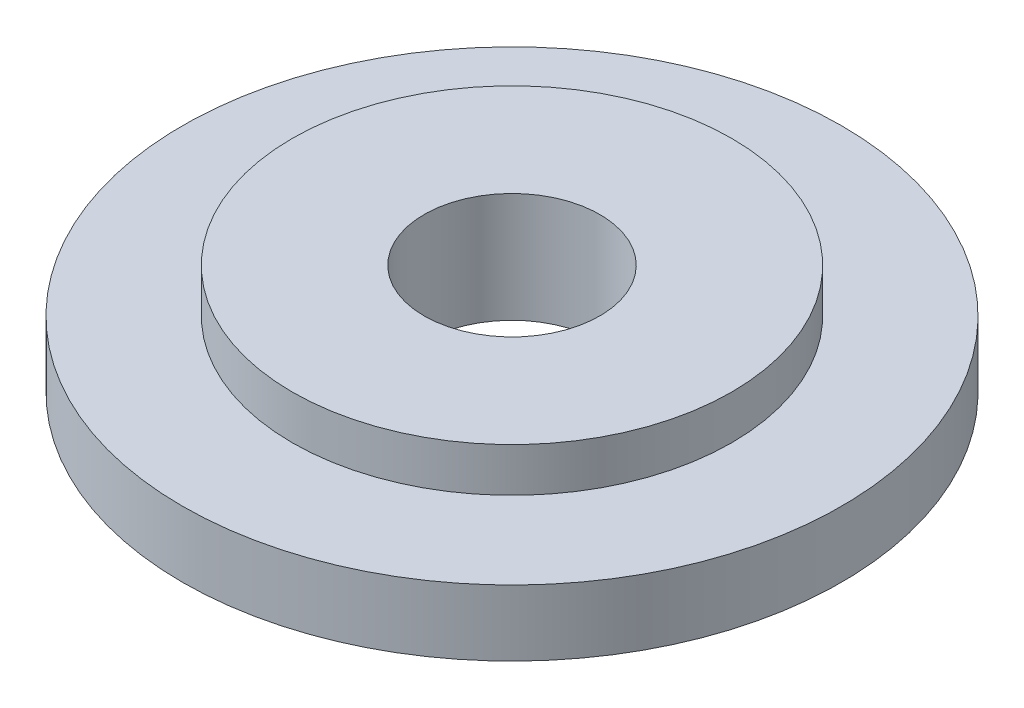
from build123d import *

# Parameters (mm, degrees)
SKETCH_1_R          = 15
EXTRUDE_1_DEPTH     = 3
SKETCH_2_R          = 10
EXTRUDE_2_DEPTH     = 2
SKETCH_3_R          = 4
CUT_EXTRUDE_1_DEPTH = 22.794494718


with BuildPart() as part:
    # 草图1 → 凸台-拉伸1 (new body)
    with BuildSketch(Plane(origin=(0, 0, 0), x_dir=(1, 0, 0), z_dir=(0, 1, 0))):
        with Locations(Location((0, 0, 0), (0, 0, 270))):
            Circle(SKETCH_1_R)
    extrude(amount=EXTRUDE_1_DEPTH)

    # 草图2 → 凸台-拉伸2 (add)
    with BuildSketch(Plane(origin=(0, 3, 0), x_dir=(1, 0, 0), z_dir=(0, 1, 0))):
        with Locations(Location((0, 0, 0), (0, 0, 270))):
            Circle(SKETCH_2_R)
    extrude(amount=EXTRUDE_2_DEPTH)

    # 草图3 → 切除-拉伸1 (cut, through all)
    with BuildSketch(Plane(origin=(0, 5, 0), x_dir=(1, 0, 0), z_dir=(0, 1, 0))):
        with Locations(Location((0, 0, 0), (0, 0, 270))):
            Circle(SKETCH_3_R)
    extrude(amount=-CUT_EXTRUDE_1_DEPTH, mode=Mode.SUBTRACT)


solid = part.part
